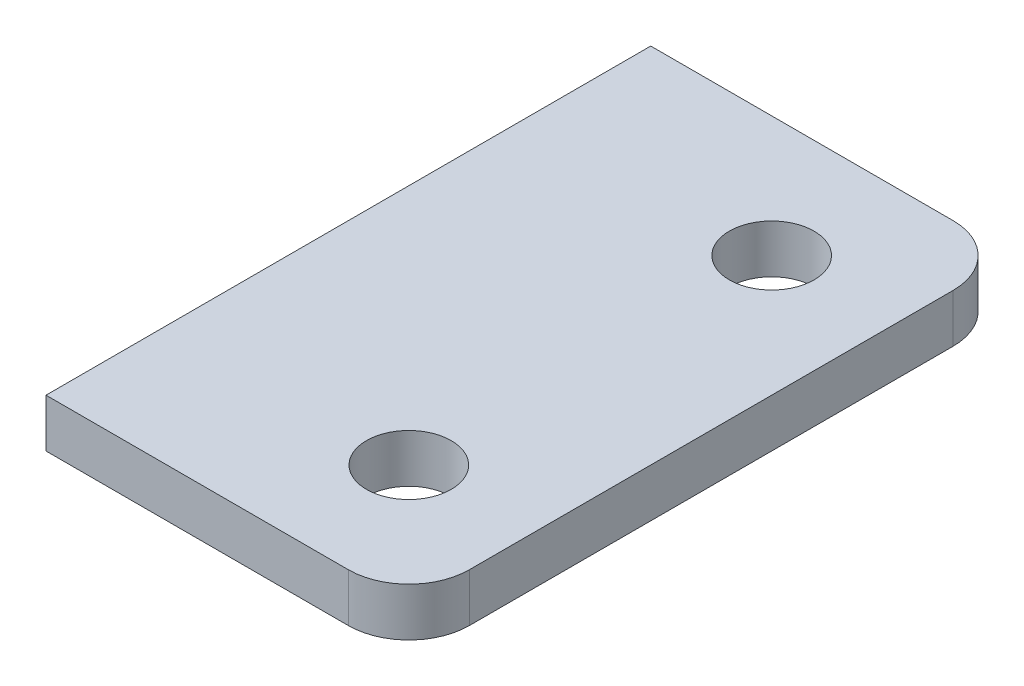
SolidWorks part; units mm, degrees
material "Q235B"
ref_plane "Front Plane" through (0, 0, 0) normal (0, 0, 1) x (1, 0, 0)
ref_plane "Top Plane" through (0, 0, 0) normal (0, 1, 0) x (1, 0, 0)
ref_plane "Right Plane" through (0, 0, 0) normal (1, 0, 0) x (0, 0, -1)
other "Configuration Table"
sketch "Sketch1" plane through (0, 0, 0) normal (0, 1, 0) x (1, 0, 0)
  line L0 (0, 0) -> (110.4251, 0) construction
  line L1 (-30, -50) -> (20, -50)
  line L2 (-30, -50) -> (-30, 50)
  line L3 (-30, 50) -> (20, 50)
  line L4 (30, -40) -> (30, 40)
  line L5 (-30, -50) -> (30, 50) construction
  line L6 (-30, 50) -> (30, -50) construction
  arc A0 (20, -50) -> (30, -40) centre (20, -40) ccw
  arc A1 (20, 50) -> (30, 40) centre (20, 40) cw
  circle A2 centre (10, 30) radius 7
  circle A3 centre (10, -30) radius 7
  point P0 (0, 0)
  dimension "D3" = 10
  dimension "D6" = 14
  dimension "D1" = 60
  dimension "D2" = 100
  dimension "D4" = 40
  dimension "D5" = 30
extrude "Boss-Extrude1" add sketch "Sketch1" along normal blind 8
